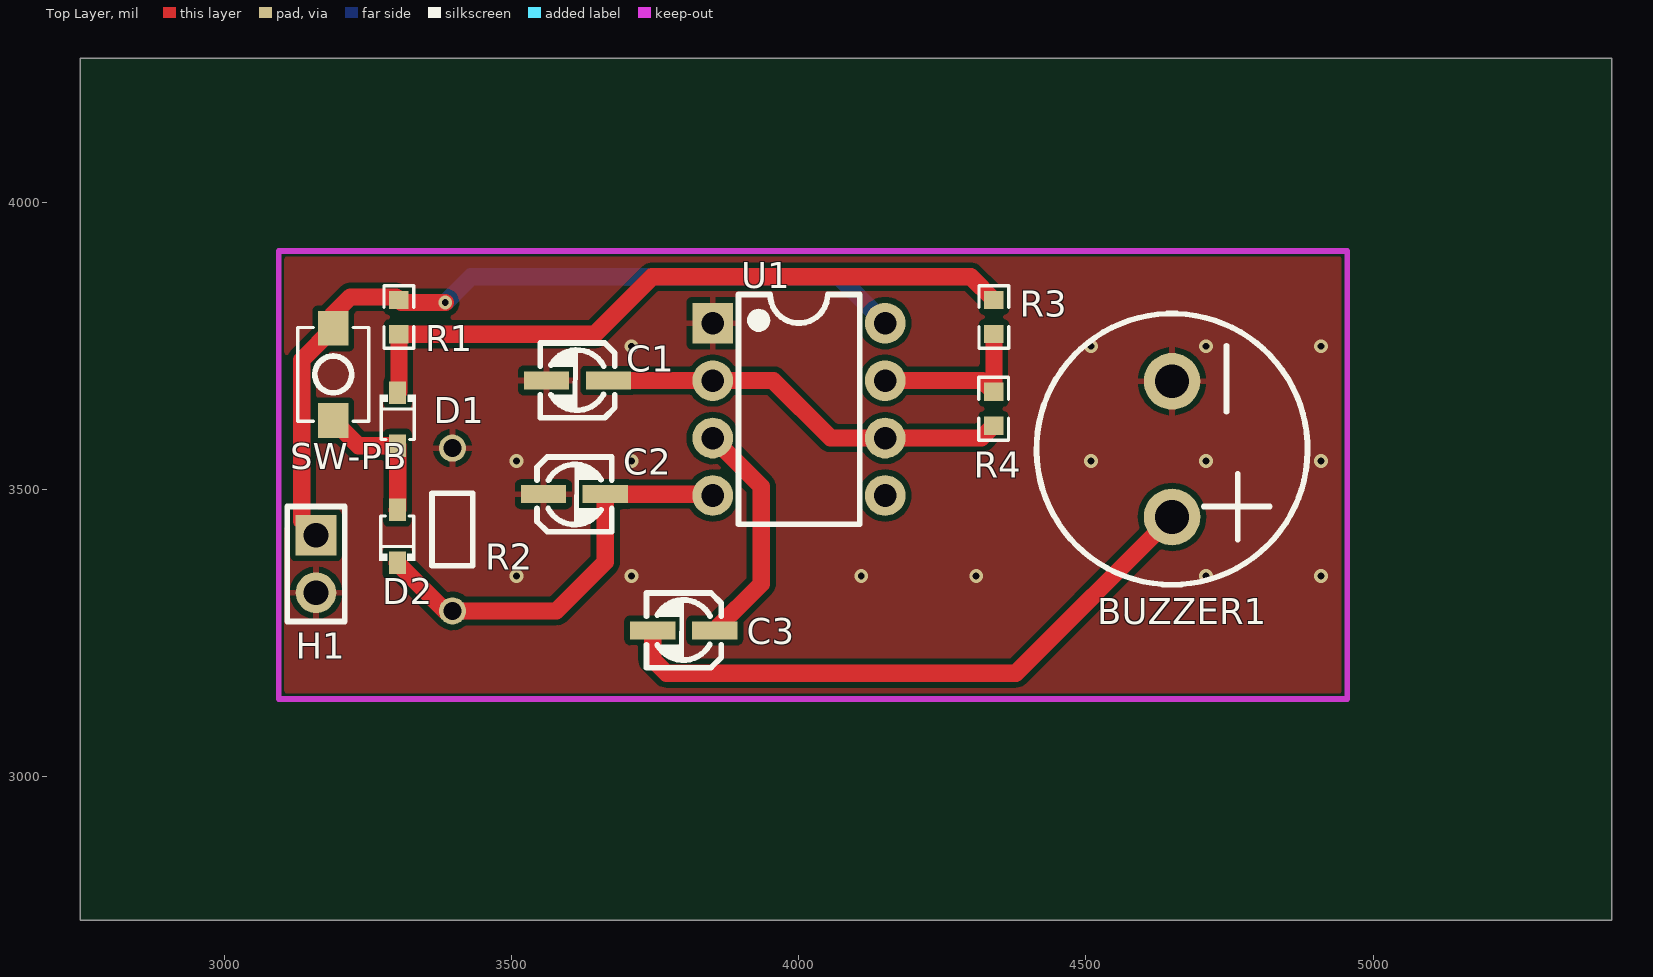
[diagram p0: Top Layer view]
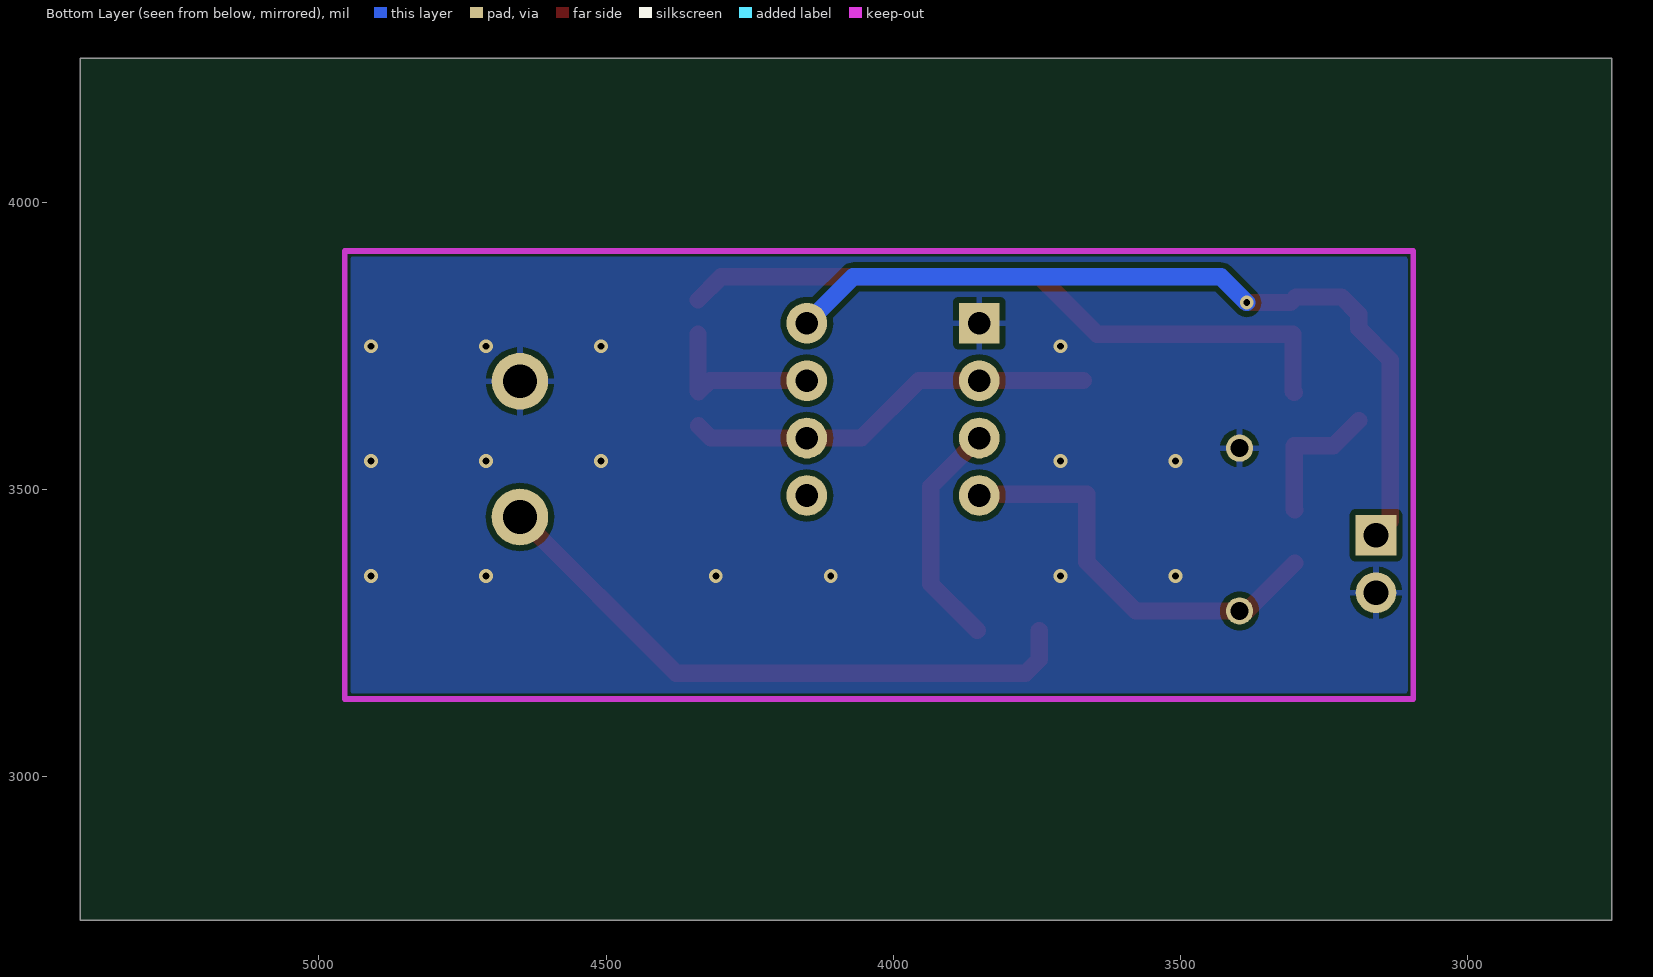
[diagram p1: Bottom Layer view, seen from below]
# Altium PCB MISC51944.pcbdoc
Units mil, origin at the board's own origin, x right, y up, seen from the top; angles counter-clockwise.
Board outline 2665 x 1500 mil, 2 copper layers (Top Layer, Bottom Layer), stack 62.206 mil thick; 13 components, 9 nets, 32 pads, 16 vias.

## Layer stack, top to bottom
Top Solder Mask Layer: solder mask 0.394, Dk 3.3
Top Layer: signal copper 1.379
Dielectric1: surface 59.449, FR4, Dk 4.5
Bottom Layer: signal copper 1.378
Bottom Solder Mask Layer: solder mask 0.394, Dk 3.3

## Board outline
5415,2750 2750,2750 2750,4250 5415,4250

## Design rules (kind name [scope] priority, off if disabled: settings)
BoardOutlineClearance copperThickness2oz_1 [All] p2 off: genericclearance=7.99 ignorepadtopadclearanceinfootprint=FALSE except(0: Arc-SplitContinuation Track-SplitContinuation SMDPad-SplitContinuation THPad-SplitContinuation Via-SplitContinuation Fill-SplitContinuation Region-SplitContinuation Poly-SplitContinuation Text-SplitContinuation Hole-SplitContinuation; 5.98: Arc-CutoutEdge SMDPad-CutoutEdge THPad-CutoutEdge Via-CutoutEdge Fill-CutoutEdge Region-CutoutEdge Text-CutoutEdge; 6.93: Hole-OutlineEdge Hole-CutoutEdge; 10: Poly-OutlineEdge Poly-CutoutEdge; 11.81: Arc-OutlineEdge Track-OutlineEdge SMDPad-OutlineEdge THPad-OutlineEdge Via-OutlineEdge Fill-OutlineEdge Region-OutlineEdge Text-OutlineEdge Track-CutoutEdge)
BoardOutlineClearance copperThickness1oz_1 [All] p4: genericclearance=4.02 ignorepadtopadclearanceinfootprint=FALSE except(0: Arc-SplitContinuation Track-SplitContinuation SMDPad-SplitContinuation THPad-SplitContinuation Via-SplitContinuation Fill-SplitContinuation Region-SplitContinuation Poly-SplitContinuation Text-SplitContinuation Hole-SplitContinuation; 6: SMDPad-CutoutEdge THPad-CutoutEdge Via-CutoutEdge Fill-CutoutEdge Region-CutoutEdge Text-CutoutEdge; 6.93: Hole-OutlineEdge Hole-CutoutEdge; 10: Poly-OutlineEdge Poly-CutoutEdge; 11.8: Arc-OutlineEdge Track-OutlineEdge SMDPad-OutlineEdge THPad-OutlineEdge Via-OutlineEdge Fill-OutlineEdge Region-OutlineEdge Text-OutlineEdge; 11.81: Arc-CutoutEdge Track-CutoutEdge)
Clearance copperThickness2oz [All] p1 off: gap=7.99 ignorepadtopadclearanceinfootprint=FALSE except(5.98: SMDPad-Track SMDPad-SMDPad THPad-Track SMDPad-THPad THPad-THPad Track-Via SMDPad-Via THPad-Via Via-Via Fill-Track Region-Track Fill-SMDPad Region-SMDPad Fill-THPad Region-THPad Fill-Via Region-Via Fill-Fill Fill-Region Region-Region Arc-Track Arc-SMDPad Arc-THPad Arc-Via Fill-Arc Region-Arc Arc-Arc Text-Track SMDPad-Text Text-THPad Text-Via Fill-Text Region-Text Arc-Text Text-Text; 6.93: Hole-Track Hole-SMDPad Hole-THPad Hole-Via Fill-Hole Region-Hole Hole-Arc Hole-Text; 10: Poly-Track Poly-SMDPad Poly-THPad Poly-Via Poly-Fill Poly-Region Poly-Poly Poly-Arc Poly-Text Poly-Hole)
Clearance copperThickness1oz [All] p3: gap=4.02 ignorepadtopadclearanceinfootprint=FALSE except(5.98: SMDPad-Track SMDPad-SMDPad THPad-Track SMDPad-THPad THPad-THPad Track-Via SMDPad-Via THPad-Via Via-Via Fill-Track Region-Track Fill-SMDPad Region-SMDPad Fill-THPad Region-THPad Fill-Via Region-Via Fill-Fill Fill-Region Region-Region; 6: Arc-Track Arc-SMDPad Arc-THPad Arc-Via Fill-Arc Region-Arc Arc-Arc Text-Track SMDPad-Text Text-THPad Text-Via Fill-Text Region-Text Arc-Text Text-Text; 6.93: Hole-Track Hole-SMDPad Hole-THPad Hole-Via Fill-Hole Region-Hole Hole-Arc Hole-Text; 10: Poly-Track Poly-SMDPad Poly-THPad Poly-Via Poly-Fill Poly-Region Poly-Poly Poly-Arc Poly-Text Poly-Hole)
DiffPairsRouting differentialPair [All] p1: maxlimit=6 minlimit=6 mostfreqgap=6 toplayer_minwidth=5 toplayer_prefwidth=10 toplayer_maxwidth=100 toplayer_mingap=6 toplayer_prefgap=6 toplayer_maxgap=6 bottomlayer_minwidth=5 bottomlayer_prefwidth=10 bottomlayer_maxwidth=100 bottomlayer_mingap=6 bottomlayer_prefgap=6 bottomlayer_maxgap=6 maxuncoupledlength=10
HoleToHoleClearance otherClearance [All] p1: gap=11.81 allowstackedmicrovias=TRUE
Length netLength [All] p1: minlimit=0 maxlimit=0
MatchedLengths netLengthTolerance [All] p1: tolerance=1000
PasteMaskExpansion pasteMaskExpansion [All] p1: expansion=0
PlaneConnect innerPlane [All] p1: planeconnectstyle=Relief reliefexpansion=20 reliefentries=4 reliefconductorwidth=10 reliefairgap=10
PolygonConnect copperRegion [(InNet('GND'))] p1: connectstyle=Relief reliefconductorwidth=10 reliefentries=4 polygonreliefangle="90 Angle" airgapwidth=10 via.connectstyle=Relief via.reliefconductorwidth=10 via.reliefentries=4 via.polygonreliefangle="90 Angle" via.airgapwidth=10
RoutingVias viaSize [All] p1: holewidth=12.01 width=24.02 viastyle="Through Hole" minholewidth=11.81 minwidth=19.68 maxholewidth=248.03 maxwidth=393.7
SolderMaskExpansion solderMaskExpansion [IsVia] p1: expansion=-1000 istentingtop=TRUE
SolderMaskExpansion solderMaskExpansion [All] p2: expansion=2 istentingtop=FALSE
Width copperThickness2oz_2 [All] p1 off: maxlimit=100 minlimit=8 preferedwidth=10
Width copperThickness1oz_2 [All] p2: maxlimit=100 minlimit=5 preferedwidth=10

## Components (designator, comment, footprint, x,y, rotation, side; value= is the part's Value field where it differs from the comment)
BUZZER1 "buzzer" BUZ-TH_BD12.0-P6.00-D0.9-RD 4650,3570 r270 top
C1 "0.01uF" C_Ele_SMD_3x5.4mm 3615,3690 r0 top
C2 "47uF" C_Ele_SMD_3x5.4mm 3609.92,3491.06 r180 top
C3 "47uF" C_Ele_SMD_3x5.4mm 3800,3255 r0 top
D1 "1N4148W" SOD-323_L1.8-W1.3-LS2.5-RD 3302.24,3622.22 r270 top
D2 "1N4148W" SOD-323_L1.8-W1.3-LS2.5-RD 3301.47,3418.08 r90 top
H1 "" HDR-TH_2P-P2.54-V-M-1 3160,3370 r270 top
R1 "30K" R0603 3304.32,3799.74 r90 top
R2 "47kΩ" Res_1/8W 3395,3430 r270 top
R3 "22K" R0603 4340,3800 r90 top
R4 "22K" R0603 4339.32,3640.2 r90 top
SW-PB "" Key_SMD_3x4x2 3190,3700 r90 top
U1 "NE555N(XBLW)" PDIP-8_L9.5-W6.4-P2.54-LS7.6-BL 4000.58,3639.25 r270 top

## Footprints (in the part's own frame and the unit in brackets; to place one, negate y for a bottom-side part, rotate by r counter-clockwise, add the part's x,y. Pads: shape width x height; smd on the part's side, far side on the other; paste and mask are expansions set on the pad)
BUZ-TH_BD12.0-P6.00-D0.9-RD [mm]
  round 2.5 hole 1.5 paste+0 mask+0.05: 1(-3,0) 2(3,0)
  silkscreen extent -5.99,-5.99 5.99,5.99
C_Ele_SMD_3x5.4mm [mil]
  rect 78.7x31.5 smd paste+0 mask+2: 1(54.1,-0.55) 2(-53.7,-0.55)
  silkscreen extent -65,-65 65,65
HDR-TH_2P-P2.54-V-M-1 [mm]
  rect 1.8x1.8 hole 1.1: 1(-1.27,0)
  round 1.8 hole 1.1: 2(1.27,0)
  silkscreen extent -2.54,-1.27 2.54,1.27
Key_SMD_3x4x2 [mm]
  rect 1.53x1.36 smd paste+0 mask+0.051: 1(-2.035,0) 2(2.035,0)
  silkscreen extent -2.08,-1.58 2.08,1.58
PDIP-8_L9.5-W6.4-P2.54-LS7.6-BL [mm]
  rect 1.8x1.8 hole 1: 1(-3.81,-3.81)
  round 1.8 hole 1: 2(-1.27,-3.81) 3(1.27,-3.81) 4(3.81,-3.81) 5(3.81,3.81) 6(1.27,3.81) 7(-1.27,3.81) 8(-3.81,3.81)
  silkscreen extent -5.08,-2.67 5.08,2.68
R0603 [mil]
  rect 31.75x34.02 smd paste-3937.01 mask+2: 1(-29.66,0) 2(29.66,0)
  silkscreen extent -55,-26 55,26
Res_1/8W [mil]
  round 47.2 hole 31.5 paste+0 mask+2: 1(-141.7,2.48) 2(141.7,2.48)
  silkscreen extent -63,-33 63,38
SOD-323_L1.8-W1.3-LS2.5-RD [mm]
  rect 1x0.75 smd: 1(-1.173,0) 2(1.173,0)
  silkscreen extent -1.08,-0.8 0.9,0.8

## Via types
v1: diameter 24.02, hole 12, Top Layer to Bottom Layer, 16 vias

## Nets (pads, with @x,y where several pads share a name; then routed paths per layer and width w, separated by ;. In a path a pad name is that pad's centre, name@x,y a point inside that pad or via, vN(x,y) a via of type N, cw(c..) or ccw(c..) an arc to the next point about the centre after c; other vN are vias at no path point)
$1N1: D1.2 D2.2 SW-PB.1 | length 242.5
  Top Layer w30: SW-PB.1 3233.82,3576.06 D1.2 3302.24,3465.02 D2.2
$1N2: D1.1 R1.1 R3.2 | length 1196.3
  Top Layer w30: D1.1 3304.32,3670.47 R1.1 3645.08,3770.08 3745,3870 4299.66,3870 R3.2
$1N3: H1.1 R1.2 SW-PB.2 U1.8 | length 1447.4
  Top Layer w30: H1.1 3135,3445 3135,3725.12 SW-PB.2 3190,3805 3220,3835 3298.72,3835 R1.2 3308.72,3825 v1(3385,3825)
  Bottom Layer w30: v1(3385,3825) 3430,3870 4069.83,3870 U1.8
$1N4: C2.2 D2.1 R2.2 U1.4 | length 738.1
  Top Layer w30: D2.1 3385.08,3288.3 R2.2 3578.3,3288.3 3663.62,3373.62 C2.2 3848.22,3491.61 U1.4
$1N10: C1.1 R4.1 U1.2 U1.6 | length 720.5
  Top Layer w30: C1.1 3850.38,3689.45 U1.2 3955.75,3689.25 4055.75,3589.25 U1.6 4318.03,3589.25 R4.1
$1N11: R3.1 R4.2 U1.7 | length 297.5
  Top Layer w30: U1.7 4319.93,3689.25 R4.2 4340,3670.54 R3.1
$1N12: C3.1 U1.3 | length 403.3
  Top Layer w30: U1.3 3935,3504.83 3935,3335.35 C3.1
$1N13: BUZZER1.2 C3.2 | length 1076.9
  Top Layer w30: C3.2 3746.3,3203.7 3770,3180 4378.11,3180 BUZZER1.2
GND: BUZZER1.1 C1.2 C2.1 H1.2 R2.1 U1.1
  other v1: 3509.1,3349.1 3709.1,3349.1 4109.1,3349.1 4309.1,3349.1 4709.1,3349.1 4909.1,3349.1 3509.1,3549.1 3709.1,3549.1 4509.1,3549.1 4709.1,3549.1 4909.1,3549.1 3709.1,3749.1 4509.1,3749.1 4709.1,3749.1 4909.1,3749.1
pads on no net: U1.5

## Polygon pours and split planes (outlines as drawn)
GND on Top Layer (solid, remove dead copper, pour order 0): 3000,4000 3000,3060 5165,3060 5165,4000
GND on Bottom Layer (solid, remove dead copper, pour order 2): 3035,3970 3035,3000 5075,3000 5075,3970

## Keep-outs
Board Outline Layer:
  lines w10: 3095,3135 3095,3915 4955,3915 4955,3135 3095,3135

## Silkscreen, mask and mechanical layers (free items; w line width, h text height)
Top Silkscreen Layer: